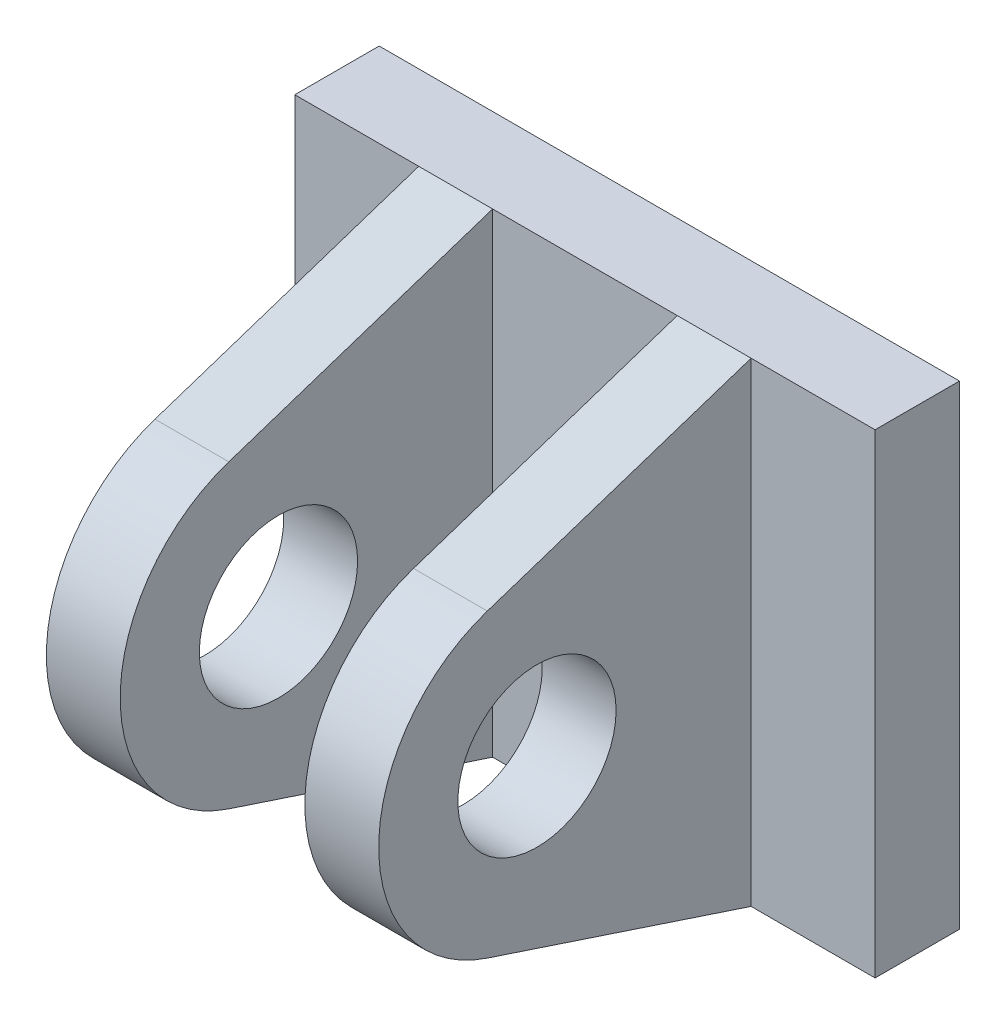
from build123d import *

# Parameters (mm, degrees)
SKETCH_1_W          = 110
SKETCH_1_H          = 90
EXTRUDE_1_DEPTH     = 16
EXTRUDE_2_DEPTH     = 14
SKETCH_3_R          = 15
CUT_EXTRUDE_1_DEPTH = 14


with BuildPart() as part:
    # 草图1 → 凸台-拉伸1 (new body)
    with BuildSketch(Plane.XY):
        Rectangle(SKETCH_1_W, SKETCH_1_H)
    extrude(amount=EXTRUDE_1_DEPTH)


with BuildPart() as body_2:
    # 草图2 → 凸台-拉伸2 (new body)
    with BuildSketch(Plane(origin=(17.5, 0, 0), x_dir=(0, 0, -1), z_dir=(1, 0, 0))):
        with BuildLine():
            Line((-16, 45), (-66, 28.486583985))
            ThreePointArc((-66, 28.486583985), (-86.591783756, 0), (-66, -28.486583985))
            Line((-66, -28.486583985), (-16, -45))
            Line((-16, -45), (-16, 45))
        make_face()
    extrude(amount=EXTRUDE_2_DEPTH)

    # 草图3 → 切除-拉伸1 (cut)
    with BuildSketch(Plane(origin=(31.5, 0, 0), x_dir=(0, 0, -1), z_dir=(1, 0, 0))):
        with Locations((-56.591783756, 0)):
            Circle(SKETCH_3_R)
    extrude(amount=-CUT_EXTRUDE_1_DEPTH, mode=Mode.SUBTRACT)


with BuildPart() as body_3:
    # 镜向1: mirrored copy
    add(body_2.part.mirror(Plane(origin=(0, 0, 0), x_dir=(0, 0, 1), z_dir=(1, 0, 0))))


solid = Compound([part.part, body_2.part, body_3.part])
